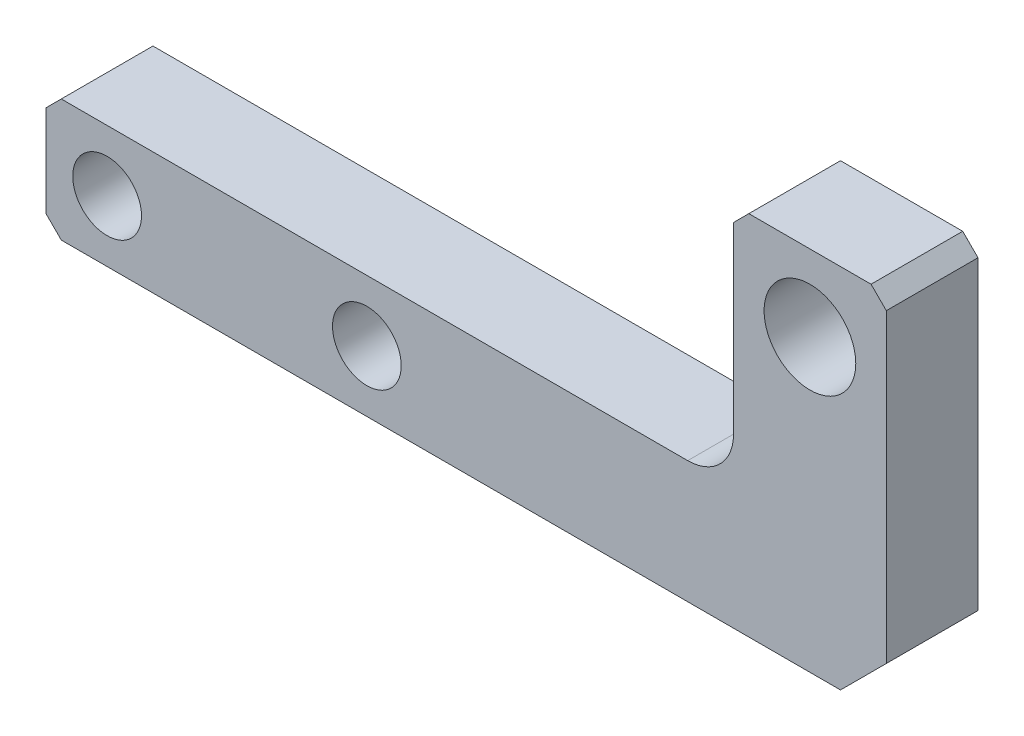
from build123d import *

# Parameters (mm, degrees)
SKETCH1_R           = 2.25
SKETCH1_R_2         = 3
BOSS_EXTRUDE1_DEPTH = 3
FILLET1_R           = 3
CHAMFER1_SIZE       = 3
CHAMFER2_SIZE       = 1


with BuildPart() as part:
    # Sketch1 → Boss-Extrude1 (new, symmetric)
    with BuildSketch(Plane.XY):
        Polygon((0, 0), (-55, 0), (-55, 8), (-10, 8), (-10, 24), (0, 24), align=None)
        with Locations((-51, 4)):
            Circle(SKETCH1_R, mode=Mode.SUBTRACT)
        with Locations((-34, 4)):
            Circle(SKETCH1_R, mode=Mode.SUBTRACT)
        with Locations((-5, 19)):
            Circle(SKETCH1_R_2, mode=Mode.SUBTRACT)
    extrude(amount=BOSS_EXTRUDE1_DEPTH, both=True)

    # Fillet1
    fillet1_edges = [part.edges().sort_by_distance(p)[0] for p in [
        (-10, 8, 0),
    ]]
    fillet(fillet1_edges, radius=FILLET1_R)

    # Chamfer1
    chamfer1_edges = [part.edges().sort_by_distance(p)[0] for p in [
        (0, 0, 0),
    ]]
    chamfer(chamfer1_edges, length=CHAMFER1_SIZE)

    # Chamfer2
    chamfer2_edges = [part.edges().sort_by_distance(p)[0] for p in [
        (-55, 0, 0),
        (-55, 8, 0),
        (-10, 24, 0),
        (0, 24, 0),
    ]]
    chamfer(chamfer2_edges, length=CHAMFER2_SIZE)


solid = part.part
